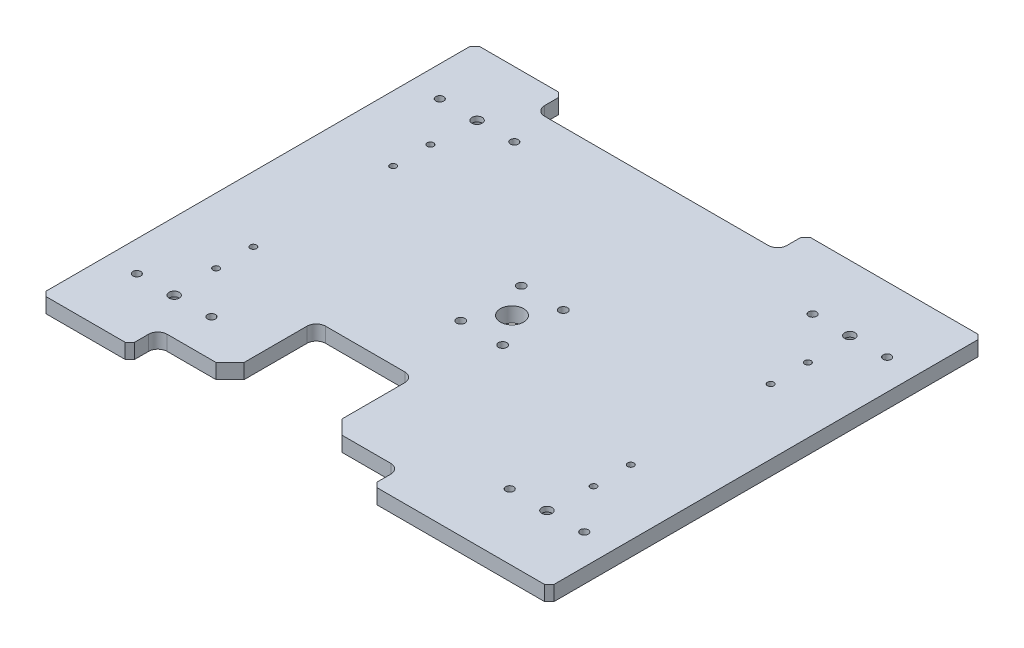
SolidWorks part; units mm, degrees
ref_plane "前视基准面" through (0, 0, 0) normal (0, 0, 1) x (1, 0, 0)
ref_plane "上视基准面" through (0, 0, 0) normal (0, 1, 0) x (1, 0, 0)
ref_plane "右视基准面" through (0, 0, 0) normal (1, 0, 0) x (0, 0, -1)
sketch "草图1" plane through (0, 0, 0) normal (0, 1, 0) x (1, 0, 0)
  line L1 (-272.5, 232.5) -> (272.5, 232.5)
  line L2 (-272.5, 232.5) -> (-272.5, -232.5)
  line L3 (-272.5, -232.5) -> (272.5, -232.5)
  line L4 (272.5, 232.5) -> (272.5, -232.5)
  line L5 (-272.5, 232.5) -> (272.5, -232.5) construction
  line L6 (-272.5, -232.5) -> (272.5, 232.5) construction
  point P0 (0, 0)
  dimension "D1" = 545
  dimension "D2" = 465
extrude "凸台-拉伸1" add sketch "草图1" along normal mid plane 16
sketch "草图2" plane through (0, 8, 0) normal (0, 1, 0) x (1, 0, 0)
  line L0 (272.5, 232.5) -> (-272.5, 232.5) construction
  line L1 (-177.5, 232.5) -> (82.5, 232.5)
  line L2 (-177.5, 232.5) -> (-177.5, 202.5)
  line L3 (-177.5, 202.5) -> (82.5, 202.5)
  line L4 (82.5, 232.5) -> (82.5, 202.5)
  line L5 (272.5, -232.5) -> (272.5, 232.5) construction
  dimension "D1" = 260
  dimension "D2" = 30
  dimension "D3" = 190
extrude "切除-拉伸1" cut sketch "草图2" against normal blind 16
mirror "镜向1" about plane through (0, 0, 0) normal (0, 0, 1) of "切除-拉伸1"
sketch "草图3" plane through (0, 8, 0) normal (0, 1, 0) x (1, 0, 0)
  line L0 (272.5, -232.5) -> (272.5, 232.5) construction
  line L1 (-100, -232.5) -> (5, -232.5)
  line L2 (-100, -232.5) -> (-100, -110)
  line L3 (-100, -110) -> (5, -110)
  line L4 (5, -232.5) -> (5, -110)
  line L6 (-177.5, -202.5) -> (82.5, -202.5) construction
  dimension "D1" = 105
  dimension "D2" = 122.5
  dimension "D3" = 267.5
  dimension "D4" = 30
extrude "切除-拉伸2" cut sketch "草图3" against normal through all
sketch "草图4" plane through (0, 8, 0) normal (0, 1, 0) x (1, 0, 0)
  circle A0 centre (200, -162.5) radius 30
  dimension "D1" = 60
  dimension "D2" = 162.5
  dimension "D3" = 200
extrude "切除-拉伸9" [suppressed] cut sketch "草图4" against normal through all
hole_wizard "M8 螺纹孔1" positions "草图6" profile "草图5" tap size "M8" standard "ISO"
sketch "草图6" [suppressed] plane through (0, 8, 0) normal (0, 1, 0) x (1, 0, 0)
  line L0 (150.2081, -162.5) -> (245.0499, -162.5) construction
  line L2 (200, -113.5579) -> (200, -210.432) construction
  circle A0 centre (200, -162.5) radius 37.5 construction
  point P12 (200, -125)
  point P14 (237.5, -162.5)
  point P16 (200, -200)
  point P18 (162.5, -162.5)
  dimension "D1" = 75
sketch "草图5" plane through (200, 8, 125) normal (1, 0, 0) x (0, 0, 1)
  line L0 (0, 0) -> (0, 16)
  line L1 (0, 16) -> (3.4, 16)
  line L2 (3.4, 16) -> (3.4, 0)
  line L5 (3.4, 0) -> (0, 0)
  line L11 (0, -6.35) -> (0, 107.95) construction
  dimension "通孔螺纹孔钻头直径" = 6.8
  dimension "通孔螺纹孔钻头深度" = 16
cosmetic thread "孔螺蚊线1" parameters "D2"=8
cosmetic thread "孔螺蚊线2" parameters "D2"=8
cosmetic thread "孔螺蚊线3" parameters "D2"=8
cosmetic thread "孔螺蚊线4" parameters "D2"=8
hole_wizard "M8 螺纹孔2" positions "草图8" profile "草图7" tap size "M8" standard "ISO" end condition through all
sketch "草图8" plane through (0, 8, 0) normal (0, 1, 0) x (1, 0, 0)
  line L0 (272.5, -232.5) -> (272.5, 232.5) construction
  point P0 (202.5, -115)
  point P2 (202.5, -75)
  dimension "D1" = 75
  dimension "D2" = 40
  dimension "D3" = 70
sketch "草图7" plane through (202.5, 8, 115) normal (1, 0, 0) x (0, 0, 1)
  line L0 (0, 0) -> (0, 16)
  line L1 (0, 16) -> (3.4, 16)
  line L2 (3.4, 16) -> (3.4, 0)
  line L5 (3.4, 0) -> (0, 0)
  line L11 (0, -6.35) -> (0, 107.95) construction
  dimension "通孔螺纹孔钻头直径" = 6.8
  dimension "通孔螺纹孔钻头深度" = 16
cosmetic thread "孔螺蚊线5" parameters "D2"=8
cosmetic thread "孔螺蚊线6" parameters "D2"=8
mirror "镜向2" about plane through (0, 0, 0) normal (1, 0, 0) of "M8 螺纹孔2", "切除-拉伸9", "M8 螺纹孔1"
mirror "镜向3" about plane through (0, 0, 0) normal (0, 0, 1) of "镜向2", "M8 螺纹孔2"
chamfer "倒角1" distance 15 angle 45 2 edges at (5, 0, 202.5) (-100, 0, 202.5)
fillet "圆角1" radius 10 6 edges at (82.5, 0, -202.5) (-177.5, 0, -202.5) (82.5, 0, 202.5) (5, 0, 110) (-100, 0, 110) (-177.5, 0, 202.5)
hole_wizard "Ø9.0 (9) 直径孔1" positions "草图11" profile "草图10" hole size "Ø9.0" standard "ISO" end condition through all
sketch "草图11" plane through (0, 8, 0) normal (0, 1, 0) x (1, 0, 0)
  line L0 (-40.7471, 0) -> (57.099, 0) construction
  point P0 (22.5, -32.5)
  point P2 (-22.5, -32.5)
  point P9 (-22.5, 32.5)
  point P10 (22.5, 32.5)
  dimension "D1" = 45
  dimension "D2" = 22.5
  dimension "D3" = 32.5
sketch "草图10" plane through (22.5, 8, 32.5) normal (1, 0, 0) x (0, 0, 1)
  line L0 (0, 0) -> (0, 16)
  line L1 (0, 16) -> (4.5, 16)
  line L2 (4.5, 16) -> (4.5, 0)
  line L5 (4.5, 0) -> (0, 0)
  line L11 (0, -6.35) -> (0, 107.95) construction
  dimension "通孔孔直径" = 9
  dimension "通孔孔深度" = 16
hole_wizard "M10 六角凹头螺钉的柱形沉头孔1" positions "草图14" profile "草图13" counterbore size "M10" standard "ISO"
sketch "草图14" plane through (0, -8, 0) normal (0, 1, 0) x (1, 0, 0)
  line L0 (0, 120.7189) -> (0, 0) construction
  line L1 (0, 0) -> (323.3002, 0) construction
  point P0 (-200, 162.5)
  point P2 (200, 162.5)
  point P4 (-200, -162.5)
  point P6 (200, -162.5)
  dimension "D1" = 400
  dimension "D2" = 325
sketch "草图13" plane through (-200, -8, -162.5) normal (1, 0, 0) x (0, 0, -1)
  line L0 (0, 0) -> (0, 27.8047)
  line L1 (0, 27.8047) -> (5.5, 24.5)
  line L2 (5.5, 24.5) -> (5.5, 10.6)
  line L3 (5.5, 10.6) -> (9, 10.6)
  line L4 (9, 10.6) -> (9, 0)
  line L5 (9, 0) -> (0, 0)
  line L10 (0, 27.8047) -> (-5.5, 24.5) construction
  line L11 (0, -6.35) -> (0, 107.95) construction
  dimension "孔直径" = 11
  dimension "孔深度" = 24.5
  dimension "柱形沉头孔直径" = 18
  dimension "柱形沉头孔深度" = 10.6
  dimension "导头角度" = 118
chamfer "倒角2" distance 5 angle 45 8 edges at (82.5, 0, 232.5) (-177.5, 0, 232.5) (82.5, 0, -232.5) (-177.5, 0, -232.5) (-272.5, 0, 232.5) (272.5, 0, 232.5) (272.5, 0, -232.5) (-272.5, 0, -232.5)
hole_wizard "M10 螺纹孔1" positions "草图16" profile "草图15" tap size "M10" standard "ISO"
sketch "草图16" plane through (0, 8, 0) normal (0, 1, 0) x (1, 0, 0)
  line L0 (-200, -162.5) -> (-200, -129.6788) construction
  line L2 (-200, -162.5) -> (-135.6571, -162.5) construction
  point P0 (-240, -162.5)
  point P2 (-160, -162.5)
  dimension "D1" = 80
sketch "草图15" plane through (-240, 8, 162.5) normal (1, 0, 0) x (0, 0, 1)
  line L0 (0, 0) -> (0, 27.0537)
  line L1 (0, 27.0537) -> (4.25, 24.5)
  line L2 (4.25, 24.5) -> (4.25, 0)
  line L5 (4.25, 0) -> (0, 0)
  line L10 (0, 27.0537) -> (-4.25, 24.5) construction
  line L11 (0, -6.35) -> (0, 107.95) construction
  dimension "螺纹孔钻头直径" = 8.5
  dimension "螺纹孔钻头深度" = 24.5
  dimension "导头角度" = 118
cosmetic thread "孔螺蚊线7" parameters "D1"=16, "D2"=10
cosmetic thread "孔螺蚊线8" parameters "D1"=16, "D2"=10
mirror "镜向4" about plane through (0, 0, 0) normal (0, 0, 1) of "M10 螺纹孔1"
mirror "镜向5" about plane through (0, 0, 0) normal (1, 0, 0) of "镜向4", "M10 螺纹孔1"
sketch "草图17" plane through (0, 8, 0) normal (0, 1, 0) x (1, 0, 0)
  circle A0 centre (0, 0) radius 12.5
  dimension "D1" = 25
extrude "切除-拉伸10" cut sketch "草图17" against normal through all
